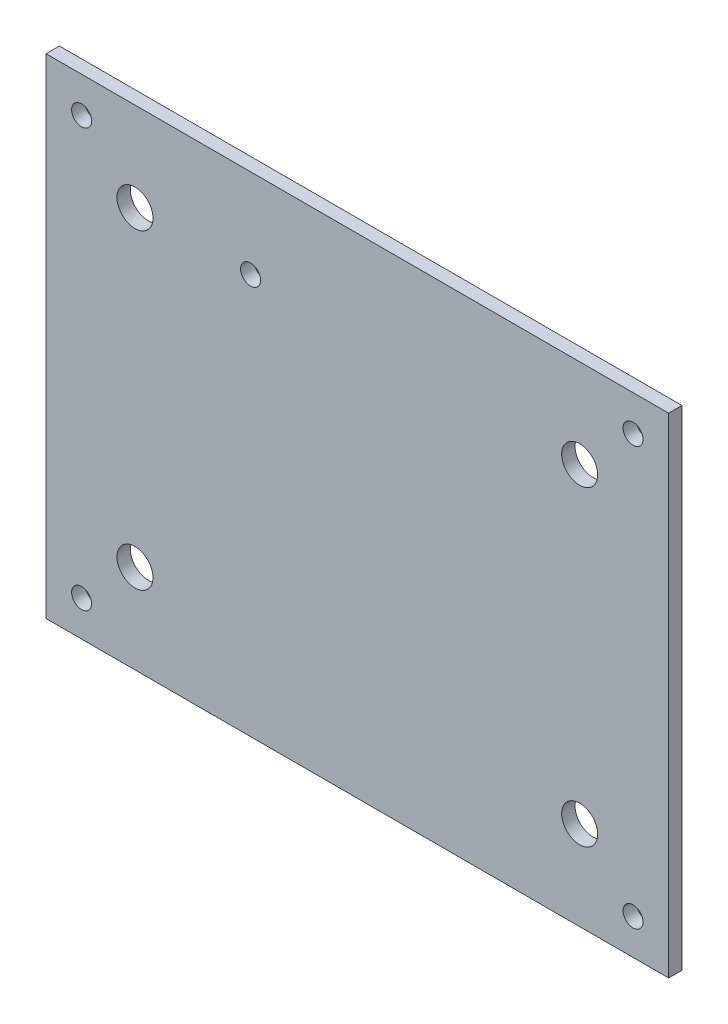
SolidWorks part; units mm, degrees
ref_plane "前视基准面" through (0, 0, 0) normal (0, 0, 1) x (1, 0, 0)
ref_plane "上视基准面" through (0, 0, 0) normal (0, 1, 0) x (1, 0, 0)
ref_plane "右视基准面" through (0, 0, 0) normal (1, 0, 0) x (0, 0, -1)
other "Configuration Table"
sketch "草图1" plane through (0, 0, 0) normal (0, 0, 1) x (1, 0, 0)
  line L0 (-70, -55) -> (70, -55)
  line L1 (70, -55) -> (70, 55)
  line L2 (70, 55) -> (-70, 55)
  line L3 (-70, 55) -> (-70, -55)
  circle A0 centre (-62, -47) radius 2.25
  circle A1 centre (-62, 47) radius 2.25
  circle A2 centre (62, -47) radius 2.25
  circle A3 centre (62, 47) radius 2.25
  circle A4 centre (-50, -35) radius 4.05
  circle A5 centre (-50, 35) radius 4.05
  circle A6 centre (50, -35) radius 4.05
  circle A7 centre (50, 35) radius 4.05
  circle A8 centre (-24, 35) radius 2.25
  point P0 (0, 0)
  dimension "D1" = 8.1
  dimension "D2" = 8.1
  dimension "D3" = 4.5
  dimension "D4" = 8.1
  dimension "D5" = 8.1
  dimension "D6" = 4.5
  dimension "D7" = 4.5
  dimension "D8" = 4.5
  dimension "D9" = 4.5
  dimension "D10" = 8
  dimension "D11" = 20
  dimension "D12" = 70
  dimension "D13" = 94
  dimension "D14" = 120
  dimension "D15" = 132
  dimension "D16" = 140
  dimension "D17" = 8
  dimension "D18" = 20
  dimension "D19" = 55
  dimension "D20" = 90
  dimension "D21" = 102
  dimension "D22" = 110
extrude "凸台-拉伸1" add sketch "草图1" against normal mid plane 3
